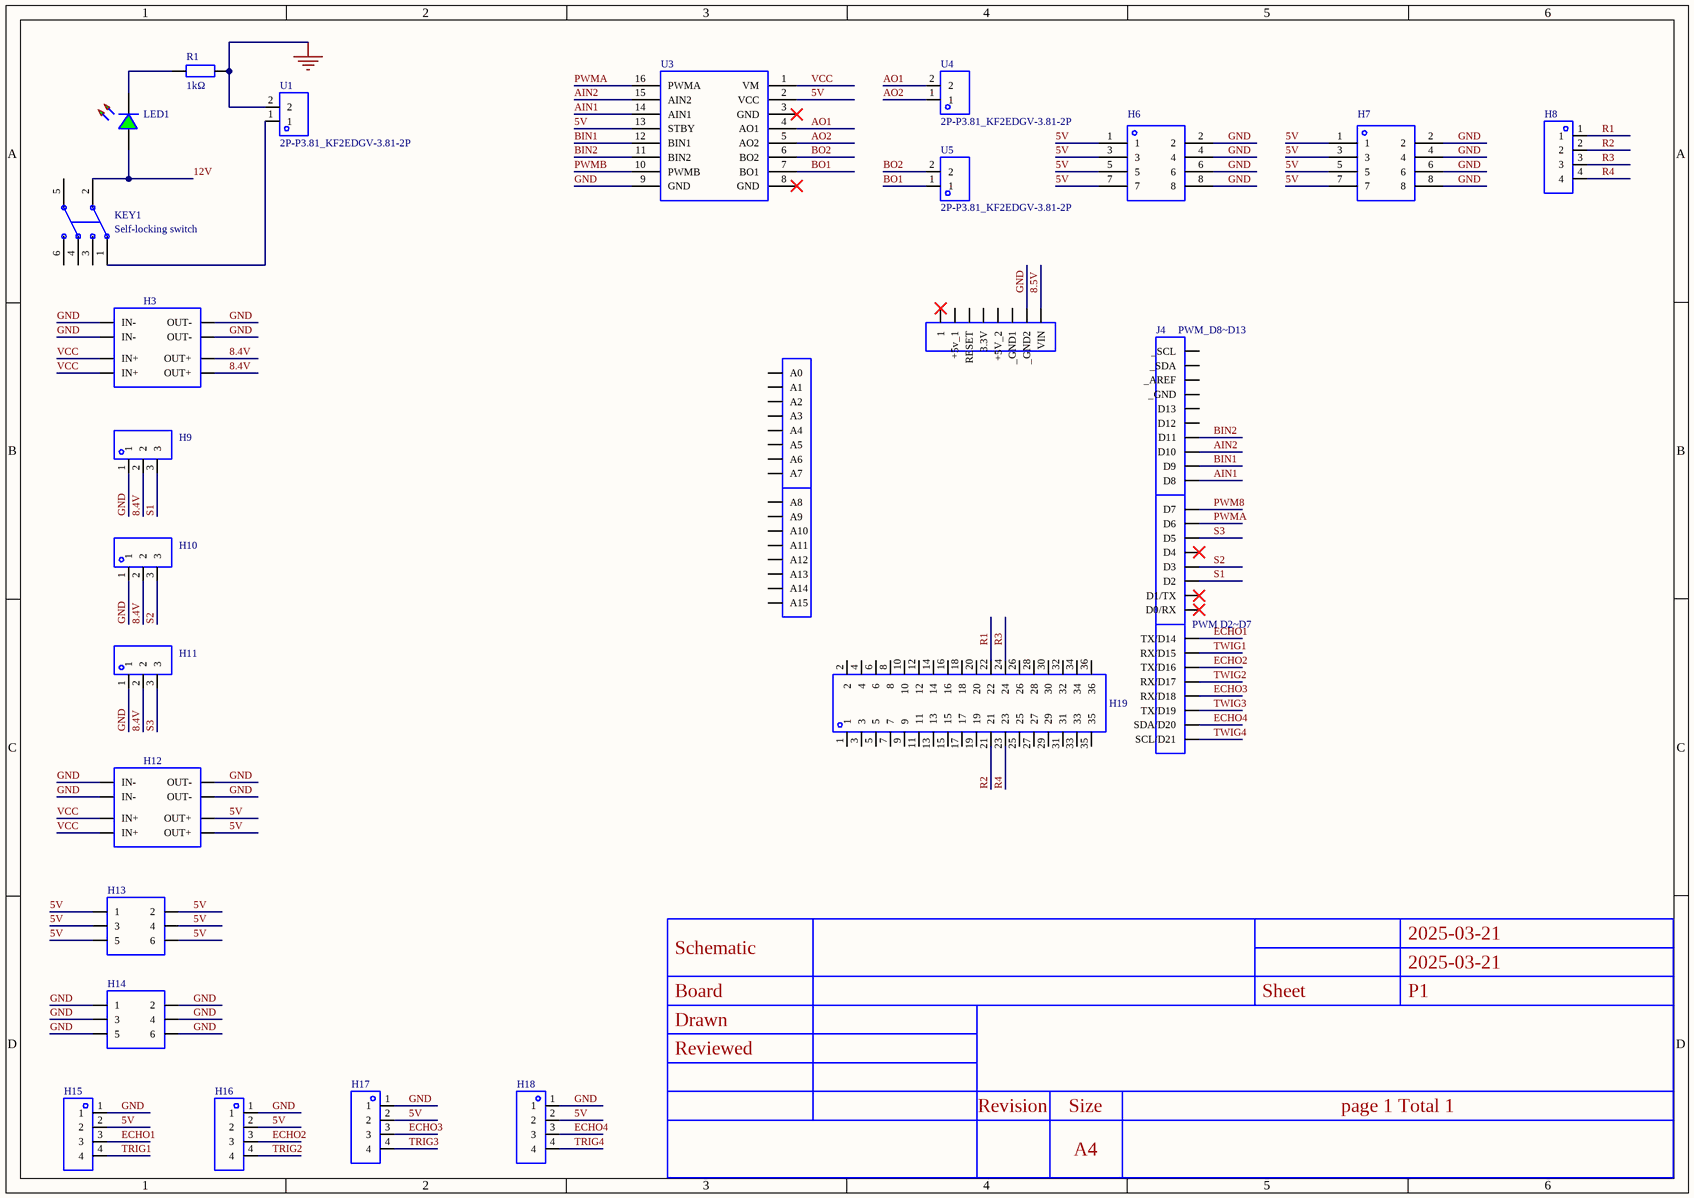
[diagram p0: MISC49940-3.schdoc]
# Altium project MISC49940-2.PrjPcb
1 sheet, 28 parts. Net scope: global (net labels, ports and power ports of the same name join across sheets).
Board file: MISC49940.pcbdoc

## Sheet MISC49940-3.schdoc
size 297 x 209 mm; Version: V1.0; @Project Name: MISC49940; @Page Count: 1; @Update Date: 2025-03-21; @Create Date: 2025-03-21; @Schematic Name: MISC49940; @Page No: 1; @Create Time: 09:51:52; @Update Time: 10:05:27; @Board Name: MISC49940

### Parts
H3  (no value)  [HDR-TH_8P-P2.54-V-M]
H6  (no value)  [HDR-TH_8P-P2.54-V-M-R2-C4-S2.54]
H7  (no value)  [HDR-TH_8P-P2.54-V-M-R2-C4-S2.54]
H8  (no value)  [HDR-TH_4P-P2.54-V-F]
H9  (no value)  [HDR-TH_3P-P2.54-V-M]
H10  (no value)  [HDR-TH_3P-P2.54-V-M]
H11  (no value)  [HDR-TH_3P-P2.54-V-M]
H12  (no value)  [HDR-TH_8P-P2.54-V-M]
H13  (no value)  [HDR-TH_6P-P2.54-V-F-R2-C3-S2.54]
H14  (no value)  [HDR-TH_6P-P2.54-V-F-R2-C3-S2.54]
H15  (no value)  [HDR-TH_4P-P2.54-V-M]
H16  (no value)  [HDR-TH_4P-P2.54-V-M]
H17  (no value)  [HDR-TH_4P-P2.54-V-M]
H18  (no value)  [HDR-TH_4P-P2.54-V-M]
H19  X6521WV-2×18H-C30D60  [HDR-TH_36P-2.54-V-M-R2-C18-S2.54]  (value not drawn)
J1  3-way TX/RX  [HDR-M-2.54_1X8]  (value not drawn)
J2  PWM D2~D7  [HDR-M-2.54_1X8]
J4  PWM_D8~D13  [HDR-M-2.54_1X10]
J8  HDR-M-2.54_1x8  [HDR-M-2.54_1X8]  (value not drawn)
J9  HDR-M-2.54_1x8  [HDR-M-2.54_1X8]  (value not drawn)
J14  HDR-M-2.54_1x8  [HDR-M-2.54_1X8]  (value not drawn)
KEY1  Self-locking switch  [SW-TH_6P-L8.5-W8.5-P2.54]
LED1  (no value)  [LED_TH-3mm]
R1  1kΩ  [Res_1/4W]
U1  2P-P3.81_KF2EDGV-3.81-2P  [CONN-TH_2P-P3.81_KF2EDGV-3.81-2P]
U3  tb6612  [tb6612]  (value not drawn)
U4  2P-P3.81_KF2EDGV-3.81-2P  [CONN-TH_2P-P3.81_KF2EDGV-3.81-2P]
U5  2P-P3.81_KF2EDGV-3.81-2P  [CONN-TH_2P-P3.81_KF2EDGV-3.81-2P]

### Nets
GND: H3.1(IN-) H3.2(IN-) H3.5(OUT-) H3.6(OUT-) H6.2 H6.4 H6.6 H6.8 H7.2 H7.4 H7.6 H7.8 H9.1 H10.1 H11.1 H12.1(IN-) H12.2(IN-) H12.5(OUT-) H12.6(OUT-) H14.1 H14.2 H14.3 H14.4 H14.5 H14.6 H15.1 H16.1 H17.1 H18.1 J9.7(_GND2) R1.2 U1.2 U3.9(GND)
5V: H6.1 H6.3 H6.5 H6.7 H7.1 H7.3 H7.5 H7.7 H12.7(OUT+) H12.8(OUT+) H13.1 H13.2 H13.3 H13.4 H13.5 H13.6 H15.2 H16.2 H17.2 H18.2 U3.2(VCC) U3.13(STBY)
8.4V: H3.7(OUT+) H3.8(OUT+) H9.2 H10.2 H11.2
8.5V: J9.8(VIN)
12V: KEY1.2 LED1.1(C)
AIN1: J4.10(D8) U3.14(AIN1)
AIN2: J4.8(D10) U3.15(AIN2)
AO1: U3.4(AO1) U4.2
AO2: U3.5(AO2) U4.1
BIN1: J4.9(D9) U3.12(BIN1)
BIN2: J4.7(D11) U3.11(BIN2)
BO1: U3.7(BO1) U5.1
BO2: U3.6(BO2) U5.2
ECHO1: H15.3 J1.1(TX/D14)
ECHO2: H16.3 J1.3(TX/D16)
ECHO3: H17.3 J1.5(RX/D18)
ECHO4: H18.3 J1.7(SDA/D20)
PWM8: J2.1(D7)
PWMA: J2.2(D6) U3.16(PWMA)
PWMB: U3.10(PWMB)
R1: H8.1 H19.22
R2: H8.2 H19.21
R3: H8.3 H19.24
R4: H8.4 H19.23
S1: H9.3 J2.6(D2)
S2: H10.3 J2.5(D3)
S3: H11.3 J2.3(D5)
TRIG1: H15.4
TRIG2: H16.4
TRIG3: H17.4
TRIG4: H18.4
TWIG1: J1.2(RX/D15)
TWIG2: J1.4(RX/D17)
TWIG3: J1.6(TX/D19)
TWIG4: J1.8(SCL/D21)
VCC: H3.3(IN+) H3.4(IN+) H12.3(IN+) H12.4(IN+) U3.1(VM)
NetKEY1_1: KEY1.1 U1.1
NetLED1_2: LED1.2(A) R1.1

Not connected (* = marked no-connect by the designer): H19 1 2 3 4 5 6 7 8 9 10 11 12 13 14 15 16 17 18 19 20 25 26 27 28 29 30 31 32 33 34 35 36; J2 4(D4)* 7(D1/TX)* 8(D0/RX)*; J4 1(_SCL) 2(_SDA) 3(_AREF) 4(_GND) 5(D13) 6(D12); J8 1(A0) 2(A1) 3(A2) 4(A3) 5(A4) 6(A5) 7(A6) 8(A7); J9 1* 2(+5v_1) 3(RESET) 4(3.3V) 5(+5V_2) 6(_GND1); J14 1(A8) 2(A9) 3(A10) 4(A11) 5(A12) 6(A13) 7(A14) 8(A15); KEY1 3 4 5 6; U3 3(GND)* 8(GND)*

### Notes on the sheet
- 2025-03-21
- Schematic
- Board
- Sheet
- P1
- Drawn
- Reviewed
- Revision
- Size
- A4
- page 1 Total 1

### Library data of the parts
H3 H12 = HDR-M_2.54_1x8P: Symbol: Header-Male-2.54_1x8; ConvertToPcb: yes; ModelId: f5b96e27511e49e38545e53df2320202; ModelTransform: 807.87244,98.425,0,0,0,0,0,0,-118.11; Device: HDR-M_2.54_1x8P; AddInBom: yes; SupplierPart: C124381; Supplier Footprint: 插件; FootprintName: HDR-TH_8P-P2.54-V-M; ModelName: HDR-TH_8P-P2.54-V-M
H6 H7 = HDR-M_2.54_2x4: Symbol: HDR-M-2.54_2x4; ConvertToPcb: yes; ModelId: 9655140a9899454ea9d6a6732d55fb0e; ModelName: HDR-TH_8P-P2.54-M-LI-2X4P; ModelTransform: 399.999,200,0,0,0,0,0,0,-118.11; Device: HDR-M_2.54_2x4; AddInBom: yes; SupplierPart: C124386; Supplier Footprint: 插件,P=2.54mm; FootprintName: HDR-TH_8P-P2.54-V-M-R2-C4-S2.54
H8 = HDR-F_2.54_1x4P: Symbol: 2.54-1*4P female; ConvertToPcb: yes; ModelId: d187812051054f85879fcaa51a310d8e; ModelTransform: 419.6842,98.464,0,0,0,0,0,0,-118.11; Device: HDR-F_2.54_1x4P; AddInBom: yes; SupplierPart: C2718488; Supplier Footprint: 插件; FootprintName: HDR-TH_4P-P2.54-V-F; ModelName: HDR-TH_4P-P2.54-V-F
H9-H11 = HDR-M_2.54_1x3P: Symbol: PZ254V-11-03P_C2937625; ConvertToPcb: yes; ModelId: bb473b6d38ff42a99216a4fcdbdcc4cb; ModelName: HDR-TH_3P-P2.54-M-LI-1X3P; ModelTransform: 299.9994,100,0,0,0,0,0,0,-118.11; Device: HDR-M_2.54_1x3P; AddInBom: yes; SupplierPart: C2937625; Supplier Footprint: 插件; FootprintName: HDR-TH_3P-P2.54-V-M
H13 H14 = HDR-F_2.54_2x3: Symbol: HDR-F-2.54_2x3; ConvertToPcb: yes; ModelId: 6dbaf143e10146ae9674d03402f6f9fb; ModelName: HDR-TH_6P-P2.54-F-LI-2X3P; ModelTransform: 315.7474,196.85,0,0,0,0,0,0,-125.984; Device: HDR-F_2.54_2x3; AddInBom: yes; SupplierPart: C92272; Supplier Footprint: 插件; FootprintName: HDR-TH_6P-P2.54-V-F-R2-C3-S2.54
H15-H18 = HDR-M_2.54_1x4P: Symbol: PZ254V-11-04P; ConvertToPcb: yes; ModelId: 112f4d05e8d64e99ab9a333894bea4f9; ModelName: HDR-TH_4P-P2.54-M-LI-1X4P; ModelTransform: 399.999,104.7242,0,0,0,0,0,0,-118.11; Device: HDR-M_2.54_1x4P; AddInBom: yes; SupplierPart: C492403; Supplier Footprint: 插件; FootprintName: HDR-TH_4P-P2.54-V-M
H19 = X6521WV-2×18H-C30D60: Manufacturer: XKB Connectivity; Convert to PCB: yes; Origin Footprint: HDR-TH_36P-2.54-V-M-R2-C18-S2.54; Device: X6521WV-2×18H-C30D60; Symbol: X6521WV-2×18H-C30D60; Add into BOM: yes; Supplier: LCSC; SupplierPart: C725890; ManufacturerPart: X6521WV-2×18H-C30D60; JLCPCB Part Class: Extended Part; FootprintName: HDR-TH_36P-2.54-V-M-R2-C18-S2.54
J1 = 3路TX/RX: Convert to PCB: yes; Origin Footprint: HDR-M-2.54_1X8; Device: 3-way TX/RX; Symbol: 3-way TX/RX; Add into BOM: yes; SupplierPart: C190820; Supplier: LCSC; FootprintName: HDR-M-2.54_1X8
J2 = PWM D2~D7: Convert to PCB: yes; Origin Footprint: HDR-M-2.54_1X8; Device: PWM D2~D7; Symbol: PWM D2~D7; Add into BOM: yes; SupplierPart: C190820; Supplier: LCSC; FootprintName: HDR-M-2.54_1X8
J4 = PWM_D8~D13: Convert to PCB: yes; Origin Footprint: HDR-M-2.54_1X10; Device: PWM_D8~D13; Symbol: PWM_D8~D13; Add into BOM: yes; SupplierPart: C57369; Supplier: LCSC; FootprintName: HDR-M-2.54_1X10
J8 J9 J14 = HDR-M-2.54_1x8: Convert to PCB: yes; Origin Footprint: HDR-M-2.54_1X8; Device: HDR-M-2.54_1x8; Symbol: HDR-M-2.54_1x8; Add into BOM: yes; SupplierPart: C190820; Supplier: LCSC; FootprintName: HDR-M-2.54_1X8
KEY1 = 无自锁开关 8.5×8.5 无声: 6脚，8.5×8.5; Manufacturer Part: 自锁开关; Symbol: No self-locking switch 8.5×8.5 silent; Device: No self-lock switch 8.5×8.5 silent; AddInBom: yes; ModelId: 4c72b3966b92446eb355e1bd0fb4f880; ModelTransform: 342.519,334.645,0,180,0,0,0,0,-137.795; Description: 6-pin, 8.5×8.5; LCSC Part Name: 无自锁开关 8.5×8.5  无声; SupplierPart: C26228; Supplier Footprint: 插件; JLCPCB Part Class: Extended library; Supplier: LCSC; ConvertToPcb: yes; FootprintName: SW-TH_6P-L8.5-W8.5-P2.54; ModelName: SW-TH_6P-L8.5-W8.5-P2.54
LED1 = LED_TH-G_3mm: ConvertToPcb: yes; ModelId: a497c992633541038a38947cdc58012f; ModelName: LED-TH-3mm_R; ModelTransform: 141.274,153.327,0,0,0,0,-5.984,0,-137.795; Device: LED_TH-G_3mm; AddInBom: yes; SymbolName: LED_TH-G; FootprintName: LED_TH-3mm; Supplier Footprint: 插件
R1 = Res_AXIAL-1/4W: AddInBom: yes; SymbolName: Resistor; ModelId: 463263665006444ab7a47bd11b0cf956; ModelName: RES-TH_BD2.4-L6.3-P10.30-D0.6; ModelTransform: 427.165,94.32816,0,0,0,0,0,0,-196.85; Value: 1kΩ; Device: Res_AXIAL-1/4W; Supplier Footprint: 轴向引线; ConvertToPcb: yes; FootprintName: Res_1/4W
U1 U4 U5 = 2P-P3.81_KF2EDGV-3.81-2P: AddInBom: yes; ModelId: d0e460b57cc144faafea3ccd6ba14e93; ModelTransform: 331.4954,283.50337,0,0,0,0,0,-23.622,-137.795; Symbol: 2P-P3.81_KF2EDGV-3.81-2P; Device: 2P-P3.81_KF2EDGV-3.81-2P; LCSC Part Name: 2P-P3.81_KF2EDGV-3.81-2P; SupplierPart: C9900017459; ManufacturerPart: 2P-P3.81_KF2EDGV-3.81-2P; Supplier Footprint: CONN-TH_2P-P3.81_KF2EDGV-3.81-2P; JLCPCB Part Class: Extended library; Supplier: LCSC; ConvertToPcb: yes; FootprintName: CONN-TH_2P-P3.81_KF2EDGV-3.81-2P; ModelName: CONN-TH_2P-P3.81_KF2EDGV-3.81-2P
U3 = tb6612: AddInBom: yes; Device: tb6612; ConvertToPcb: yes; JLCPCB Part Class: Extended library; SymbolName: tb6612; FootprintName: tb6612